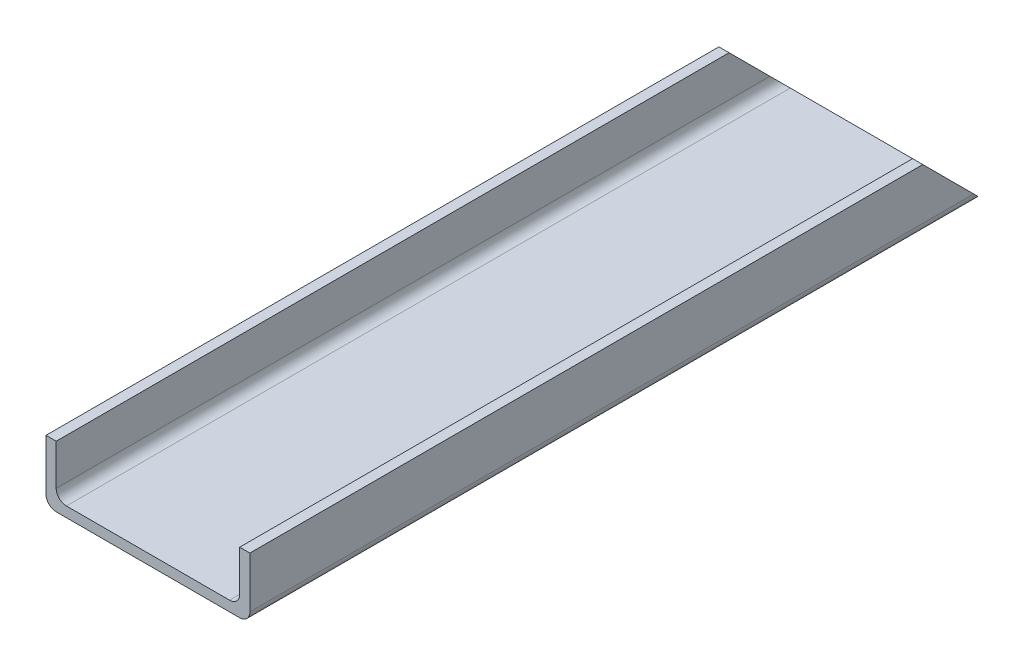
SolidWorks part; units mm, degrees
ref_plane "前视基准面" through (0, 0, 0) normal (0, 0, 1) x (1, 0, 0)
ref_plane "上视基准面" through (0, 0, 0) normal (0, 1, 0) x (1, 0, 0)
ref_plane "右视基准面" through (0, 0, 0) normal (1, 0, 0) x (0, 0, -1)
sketch "草图1" plane through (0, 0, 0) normal (0, 0, 1) x (1, 0, 0)
  line L0 (5, 0) -> (95, 0)
  line L1 (100, 5) -> (100, 30)
  line L2 (0, 5) -> (0, 30)
  line L3 (5, 10) -> (5, 30)
  line L4 (10, 5) -> (90, 5)
  line L5 (95, 10) -> (95, 30)
  line L6 (0, 30) -> (5, 30)
  line L7 (95, 30) -> (100, 30)
  line L8 (0, 0) -> (100, 0) construction
  line L9 (100, 0) -> (100, 30) construction
  line L10 (5, 5) -> (95, 5) construction
  line L11 (95, 5) -> (95, 30) construction
  line L12 (0, 0) -> (0, 30) construction
  line L13 (5, 5) -> (5, 30) construction
  arc A0 (95, 0) -> (100, 5) centre (95, 5) ccw
  arc A1 (90, 5) -> (95, 10) centre (90, 10) ccw
  arc A2 (5, 0) -> (0, 5) centre (5, 5) cw
  arc A3 (10, 5) -> (5, 10) centre (10, 10) cw
  dimension "D2" = 5
  dimension "D1" = 5
extrude "凸台-拉伸1" add sketch "草图1" along normal blind 360
sketch "草图2" plane through (0, 0, 0) normal (-1, 0, 0) x (0, 0, 1)
  line L0 (51.0969, 61.4735) -> (51.0969, 13.5445)
  line L1 (51.0969, 13.5445) -> (12.5613, -24.991)
  line L2 (38.5355, 86.4645) -> (38.5355, 38.5355)
  line L3 (38.5355, 38.5355) -> (0, 0)
  line L4 (0, 30) -> (0, 0)
  line L5 (0, 30) -> (30, 30)
  line L6 (360, 30) -> (0, 30) construction
  line M9 (0, 30) -> (0, 5)
  line M10 (0, 5) -> (360, 5)
  line M12 (360, 30) -> (0, 30)
extrude "切除-拉伸1" cut sketch "草图2" against normal through all contours L3 M12 M9 M10 | L4 L3 M10
